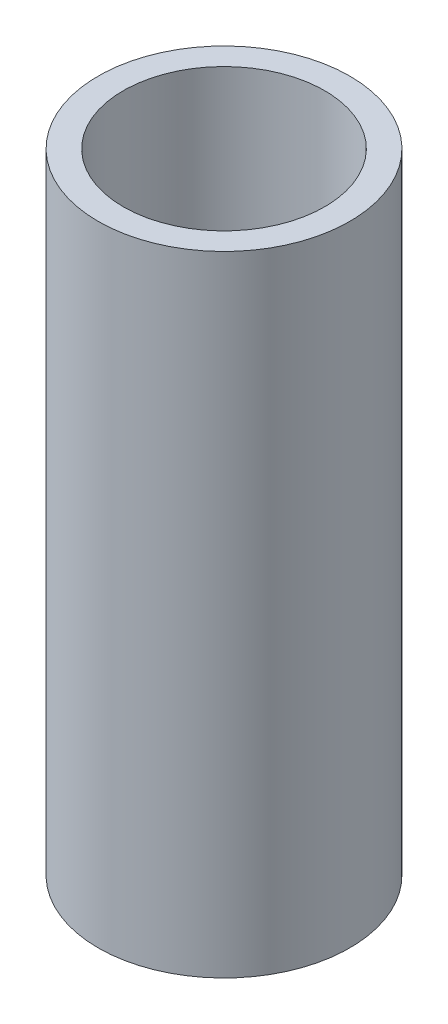
SolidWorks part; units mm, degrees
ref_plane "Front Plane" through (0, 0, 0) normal (0, 0, 1) x (1, 0, 0)
ref_plane "Top Plane" through (0, 0, 0) normal (0, 1, 0) x (1, 0, 0)
ref_plane "Right Plane" through (0, 0, 0) normal (1, 0, 0) x (0, 0, -1)
sketch "Sketch1" plane through (0, 0, 0) normal (0, 1, 0) x (1, 0, 0)
  circle A0 centre (0, 0) radius 10
  circle A1 centre (0, 0) radius 8
  dimension "D1" = 20
  dimension "D2" = 16
extrude "Boss-Extrude1" add sketch "Sketch1" along normal blind 50
